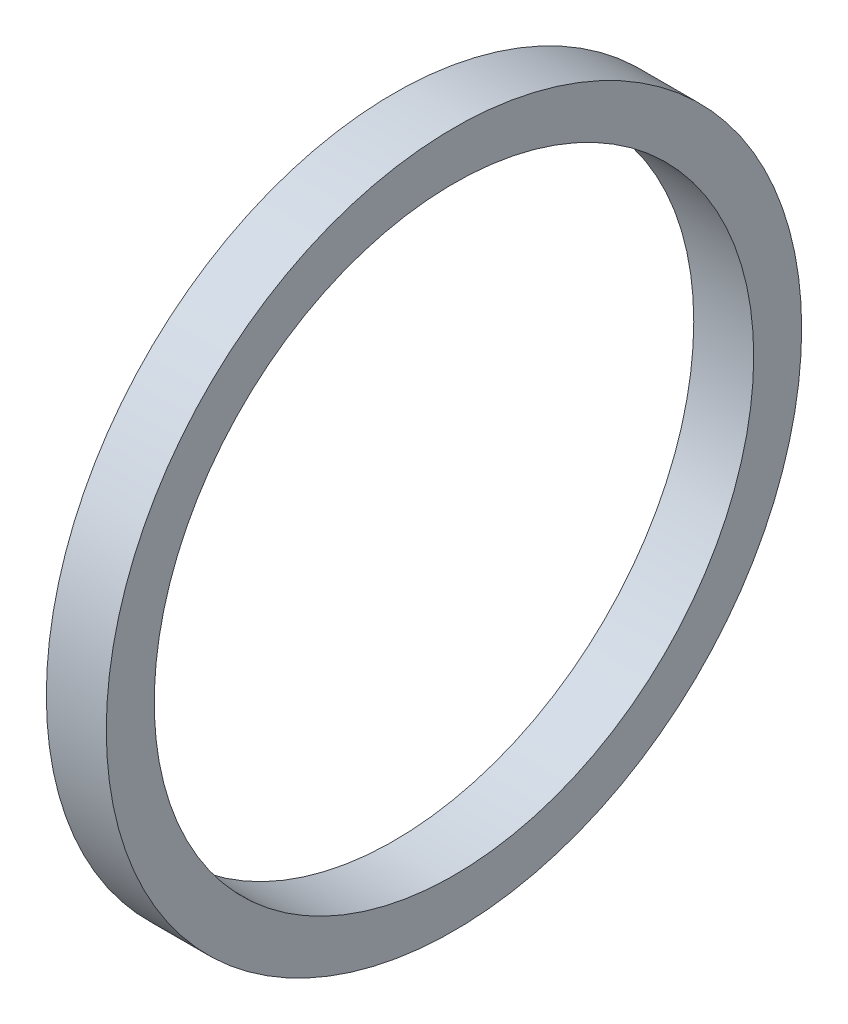
SolidWorks part; units mm, degrees
ref_plane "Front Plane" through (0, 0, 0) normal (0, 0, 1) x (1, 0, 0)
ref_plane "Top Plane" through (0, 0, 0) normal (0, 1, 0) x (1, 0, 0)
ref_plane "Right Plane" through (0, 0, 0) normal (1, 0, 0) x (0, 0, -1)
other "Configuration Table"
sketch "Sketch1" plane through (0, 0, 0) normal (1, 0, 0) x (0, 0, -1)
  circle A0 centre (0, 0) radius 20.3
  circle A1 centre (0, 0) radius 17.5
  dimension "D1" = 40.6
  dimension "D2" = 35
extrude "Boss-Extrude1" add sketch "Sketch1" along normal blind 3.5
